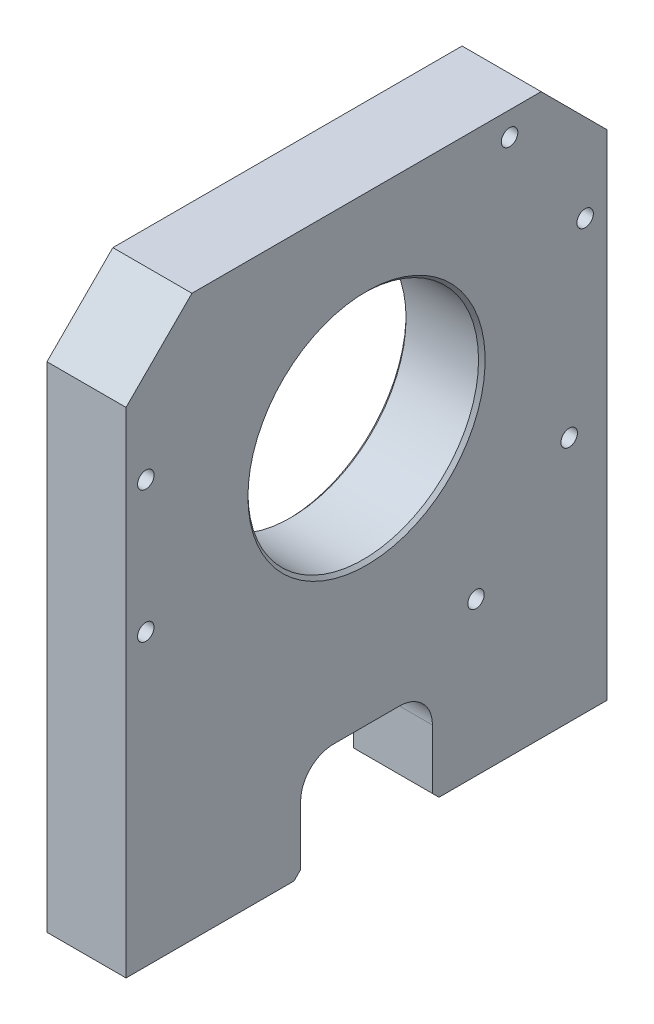
SolidWorks part; units mm, degrees
material "S45C"
ref_plane "Front Plane" through (0, 0, 0) normal (0, 0, 1) x (1, 0, 0)
ref_plane "Top Plane" through (0, 0, 0) normal (0, 1, 0) x (1, 0, 0)
ref_plane "Right Plane" through (0, 0, 0) normal (1, 0, 0) x (0, 0, -1)
sketch "Sketch1" plane through (0, 0, 0) normal (1, 0, 0) x (0, 0, -1)
  line L0 (0, 0) -> (0, 26.6506) construction
  line L1 (-36.5, 0) -> (-10, 0)
  line L2 (-36.5, 0) -> (-36.5, 85)
  line L3 (-36.5, 85) -> (36.5, 85)
  line L4 (36.5, 0) -> (36.5, 85)
  line L6 (-10, 0) -> (-10, 10)
  line L7 (-5, 15) -> (5, 15)
  line L8 (10, 0) -> (10, 10)
  line L9 (10, 0) -> (36.5, 0)
  circle A0 centre (0, 54) radius 17.5
  arc A1 (5, 15) -> (10, 10) centre (5, 10) cw
  arc A2 (-10, 10) -> (-5, 15) centre (-5, 10) cw
  point P15 (10, 15)
  point P18 (-10, 15)
  dimension "D3" = 35
  dimension "D4" = 54
  dimension "D7" = 5
  dimension "D1" = 85
  dimension "D2" = 73
  dimension "D5" = 20
  dimension "D6" = 15
extrude "Boss-Extrude1" add sketch "Sketch1" along normal mid plane 12
chamfer "Chamfer1" distance 10 angle 45 2 edges at (0, 85, 36.5) (0, 85, -36.5)
hole_wizard "M6 Tapped Hole1" positions "Sketch3" profile "Sketch2" tap size "M6" standard "Gb"
sketch "Sketch3" plane through (0, 0, 0) normal (0, -1, 0) x (-1, 0, 0)
  line L0 (23.81, 0) -> (-31.1369, 0) construction
  point P0 (0, -25)
  point P2 (0, 25)
  dimension "D1" = 50
sketch "Sketch2" plane through (0, 0, 25) normal (1, 0, 0) x (0, 0, -1)
  line L0 (0, 0) -> (0, 18.5022)
  line L1 (0, 18.5022) -> (2.5, 17)
  line L2 (2.5, 17) -> (2.5, 0)
  line L5 (2.5, 0) -> (0, 0)
  line L10 (0, 18.5022) -> (-2.5, 17) construction
  line L11 (0, -6.35) -> (0, 107.95) construction
  dimension "螺纹孔钻头直径" = 5
  dimension "螺纹孔钻头深度" = 17
  dimension "导头角度" = 118
cosmetic thread "Cosmetic Thread1" parameters "D1"=12, "D2"=6
cosmetic thread "Cosmetic Thread2" parameters "D1"=12, "D2"=6
sketch "Sketch8" plane through (0, 0, 0) normal (0, -1, 0) x (1, 0, 0)
  line L0 (0, 15.5) -> (0, 14.5) construction
  line L1 (2, 15.5) -> (2, 14.5)
  line L2 (-2, 15.5) -> (-2, 14.5)
  line L3 (-18.1924, 0) -> (18.8842, 0) construction
  circle A0 centre (0, -15) radius 2
  arc A1 (2, 15.5) -> (-2, 15.5) centre (0, 15.5) ccw
  arc A2 (-2, 14.5) -> (2, 14.5) centre (0, 14.5) ccw
  point P5 (0, 15)
  dimension "D1" = 30
  dimension "D2" = 4
  dimension "D3" = 1
extrude "Cut-Extrude1" cut sketch "Sketch8" against normal blind 15
chamfer "Chamfer2" distance 1 angle 45 2 edges at (0, 0, 10) (0, 0, -10)
hole_wizard "M3 Tapped Hole1" positions "Sketch7" profile "Sketch6" tap size "M3" standard "GB" end condition through all
sketch "Sketch7" plane through (-6, 0, 0) normal (-1, 0, 0) x (0, 0, 1)
  line L0 (0, 54) -> (41.1297, 54) construction
  line L3 (36.5, 75) -> (36.5, 0) construction
  line L4 (-33.1774, 65.0233) -> (-21.7058, 81.4063) construction
  line L7 (-30.7591, 37.383) -> (-16.617, 23.2409) construction
  line L10 (0, 54) -> (-38.4642, 15.5358) construction
  line L13 (0, 54) -> (-40.2585, 82.1893) construction
  point P0 (33.5, 44)
  point P2 (33.5, 64)
  point P20 (-16.617, 23.2409)
  point P22 (-30.7591, 37.383)
  point P24 (-33.1774, 65.0233)
  point P26 (-21.7058, 81.4063)
  dimension "D1" = 20
  dimension "D2" = 3
  dimension "D3" = 145
  dimension "D4" = 33.5
  dimension "D5" = 33.5
  dimension "D6" = 135
  dimension "D7" = 20
  dimension "D8" = 20
cosmetic thread "Cosmetic Thread3" parameters "D2"=3
cosmetic thread "Cosmetic Thread4" parameters "D2"=3
sketch "Sketch6" plane through (-6, 44, 33.5) normal (0, 1, 0) x (0, 0, 1)
  line L0 (0, 0) -> (0, 12)
  line L1 (0, 12) -> (1.25, 12)
  line L2 (1.25, 12) -> (1.25, 0)
  line L5 (1.25, 0) -> (0, 0)
  line L11 (0, -6.35) -> (0, 107.95) construction
  dimension "通孔螺纹孔钻头直径" = 2.5
  dimension "通孔螺纹孔钻头深度" = 12
cosmetic thread "Cosmetic Thread5" parameters "D2"=3
cosmetic thread "Cosmetic Thread6" parameters "D2"=3
cosmetic thread "Cosmetic Thread7" parameters "D2"=3
cosmetic thread "Cosmetic Thread8" parameters "D2"=3
chamfer "Chamfer3" distance 0.5 angle 45 2 edges at (-6, 54, -17.5) (6, 54, -17.5)
